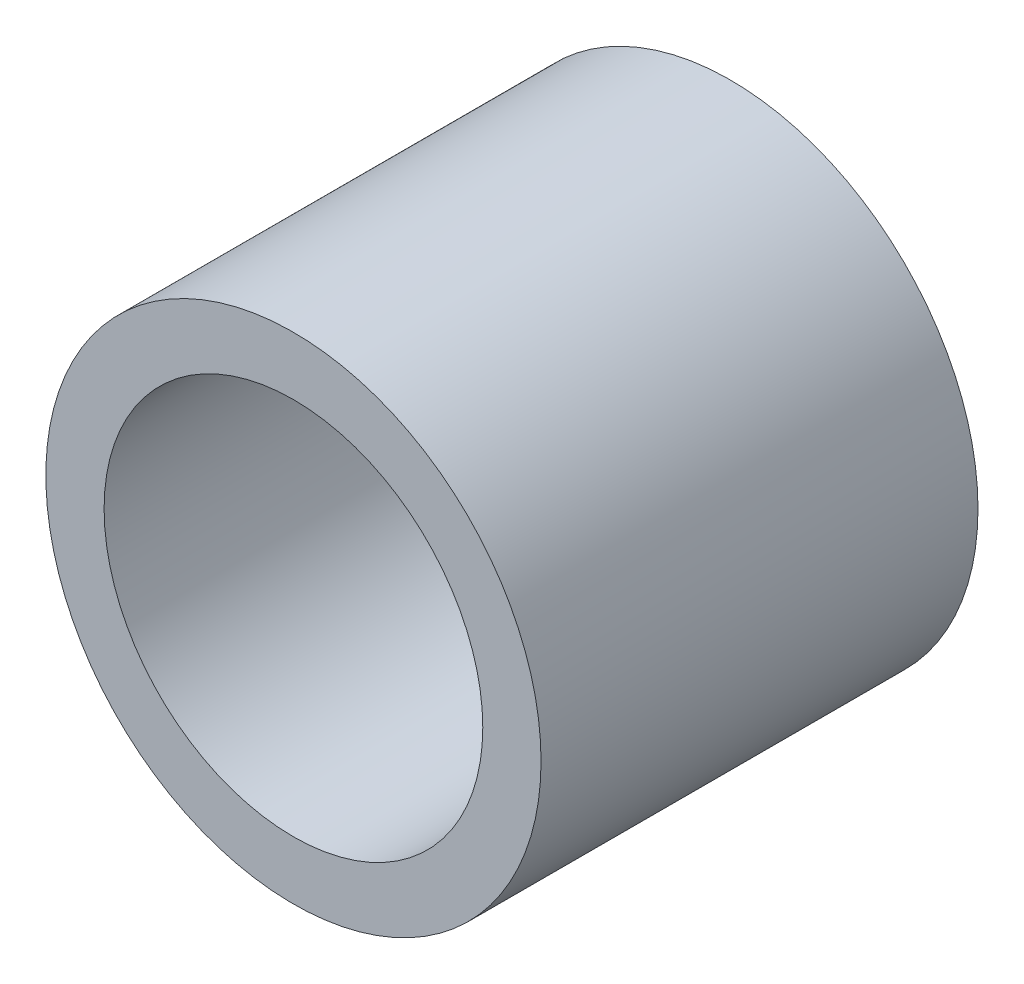
from build123d import *

# Parameters (mm, degrees)
SKETCH_1_R      = 34
SKETCH_1_R_2    = 26
EXTRUDE_1_DEPTH = 60


with BuildPart() as part:
    # 草图1 → 凸台-拉伸1 (new body)
    with BuildSketch(Plane.XY):
        Circle(SKETCH_1_R)
        Circle(SKETCH_1_R_2, mode=Mode.SUBTRACT)
    extrude(amount=EXTRUDE_1_DEPTH)


solid = part.part
